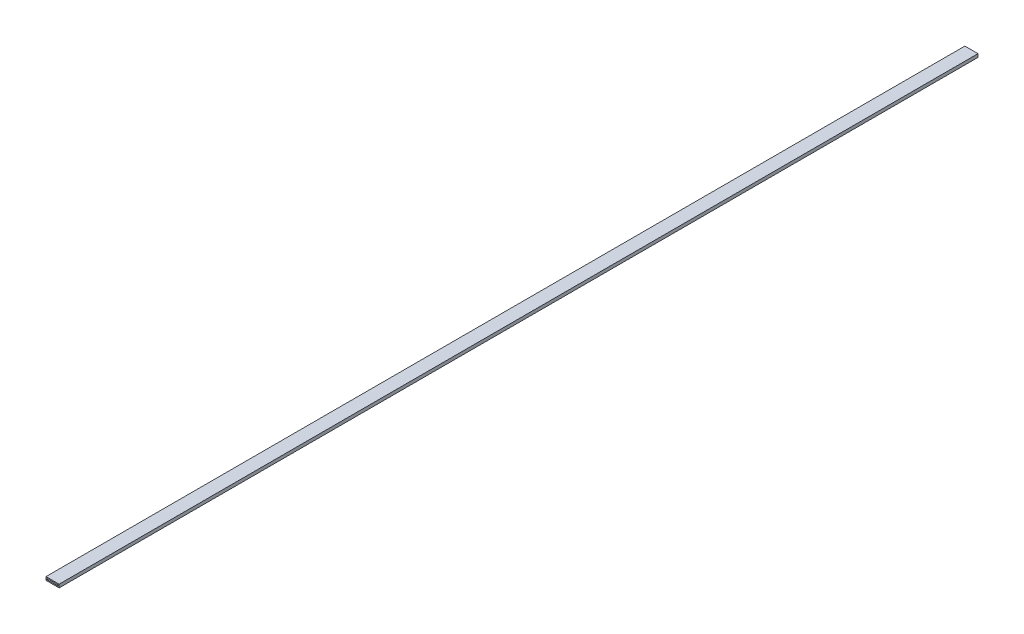
SolidWorks part; units mm, degrees
ref_plane "Front Plane" through (0, 0, 0) normal (0, 0, 1) x (1, 0, 0)
ref_plane "Top Plane" through (0, 0, 0) normal (0, 1, 0) x (1, 0, 0)
ref_plane "Right Plane" through (0, 0, 0) normal (1, 0, 0) x (0, 0, -1)
other "Configuration Table"
sketch "Sketch1" plane through (0, 0, 0) normal (0, 0, 1) x (1, 0, 0)
  line L0 (-31.901, 24.1249) -> (-19.901, 24.1249)
  line L1 (-19.901, 24.1249) -> (-19.901, 21.1249)
  line L2 (-19.901, 21.1249) -> (-31.901, 21.1249)
  line L3 (-31.901, 21.1249) -> (-31.901, 24.1249)
  dimension "D1" = 12
  dimension "D2" = 3
extrude "Boss-Extrude1" add sketch "Sketch1" along normal blind 840
sketch "Sketch2" plane through (0, 0, 840) normal (0, 0, 1) x (1, 0, 0)
  line L0 (-30.901, 23.1249) -> (-20.901, 23.1249)
  line L1 (-20.901, 23.1249) -> (-20.901, 22.1249)
  line L2 (-20.901, 22.1249) -> (-30.901, 22.1249)
  line L3 (-30.901, 22.1249) -> (-30.901, 23.1249)
  line L4 (-19.901, 24.1249) -> (-31.901, 24.1249) construction
  line L5 (-19.901, 21.1249) -> (-19.901, 24.1249) construction
  line L6 (-31.901, 21.1249) -> (-19.901, 21.1249) construction
  line L7 (-31.901, 24.1249) -> (-31.901, 21.1249) construction
  dimension "D1" = 1
  dimension "D2" = 1
  dimension "D3" = 1
  dimension "D4" = 1
extrude "Cut-Extrude1" cut sketch "Sketch2" against normal through all
sketch "Sketch3" plane through (0, 24.1249, 0) normal (0, 1, 0) x (1, 0, 0)
  line L0 (-19.901, -420) -> (-31.901, -420) construction
  line L1 (-19.901, -840) -> (-19.901, 0) construction
  line L2 (-31.901, -840) -> (-31.901, 0) construction
  line L3 (-25.901, -420) -> (-25.901, -389)
  line L4 (-25.901, -389) -> (-25.901, -451)
